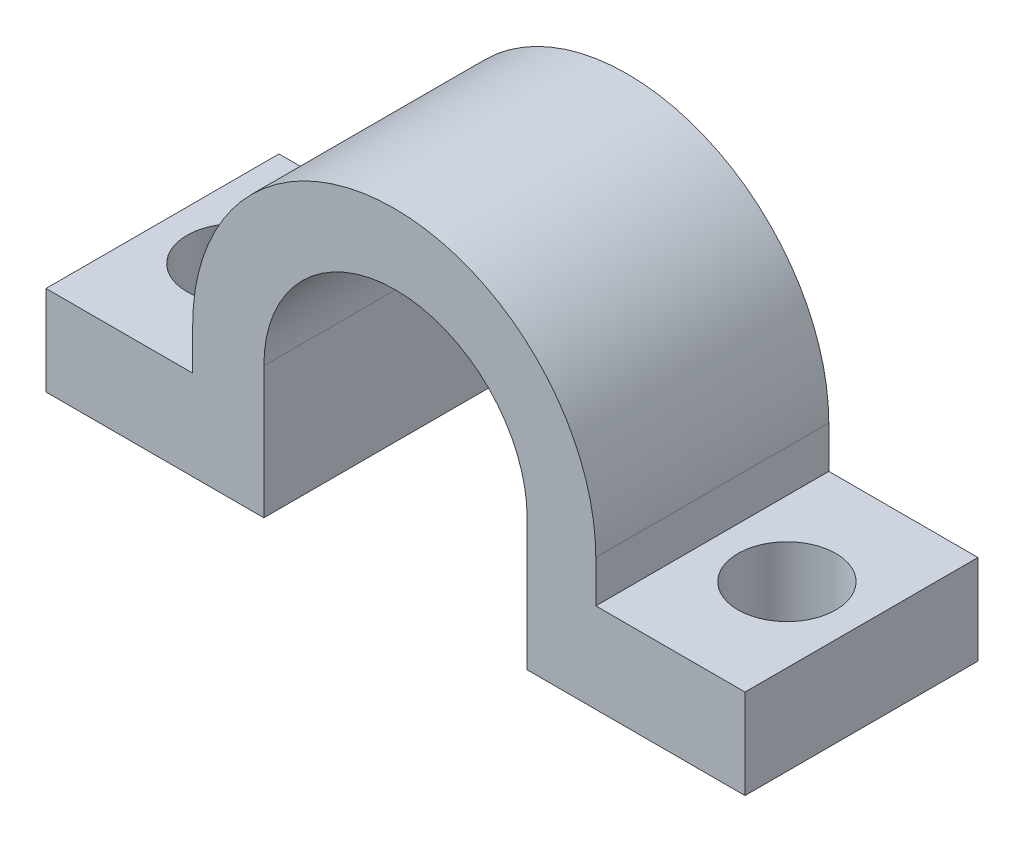
SolidWorks part; units mm, degrees
ref_plane "前视基准面" through (0, 0, 0) normal (0, 0, 1) x (1, 0, 0)
ref_plane "上视基准面" through (0, 0, 0) normal (0, 1, 0) x (1, 0, 0)
ref_plane "右视基准面" through (0, 0, 0) normal (1, 0, 0) x (0, 0, -1)
sketch "草图1" plane through (0, 0, 0) normal (0, 0, 1) x (1, 0, 0)
  line L0 (-5.5967, 5.1851) -> (-5.5967, 6.9851)
  line L13 (-14.9467, 5.1851) -> (-8.65, 5.1851)
  line L14 (-14.9467, 5.1851) -> (-14.9467, 1.3351)
  line L15 (-14.9467, 1.3351) -> (-5.5967, 1.3351)
  line L16 (-5.5967, 5.1851) -> (-5.5967, 1.3351)
  line L17 (8.65, 5.1851) -> (15.0533, 5.1851)
  line L18 (5.7033, 5.1851) -> (5.7033, 1.3351)
  line L19 (5.7033, 1.3351) -> (15.0533, 1.3351)
  line L20 (15.0533, 5.1851) -> (15.0533, 1.3351)
  line L22 (5.7033, 6.9851) -> (5.7033, 5.1851)
  line L23 (-8.65, 6.9851) -> (-8.65, 5.1851)
  line L24 (8.65, 6.9851) -> (8.65, 5.1851)
  arc A3 (8.65, 6.9851) -> (-8.65, 6.9851) centre (0, 6.9851) ccw
  arc A4 (5.7033, 6.9851) -> (-5.5967, 6.9851) centre (0.0533, 6.9851) ccw
  dimension "D1" = 3.85
  dimension "D8" = 11.3
  dimension "D2" = 3.85
  dimension "D3" = 0
  dimension "D4" = 11.3
  dimension "D6" = 9.35
  dimension "D7" = 30
extrude "凸台-拉伸1" add sketch "草图1" along normal blind 10
extrude "切除-拉伸1" cut sketch "草图2" against normal up to surface (17.7 mm away)
sketch "草图2" plane through (-970.0906, 5.1851, 1019.2503) normal (0, 1, 0) x (0, 0, 1)
  line L0 (-1055.2503, 985.1439) -> (-1055.2503, 955.1439) construction
  line L3 (-1014.2503, 985.1439) -> (-1014.2503, 955.1439) construction
  line L6 (-1060.2503, 981.9423) -> (-1009.2503, 981.9423) construction
  line L9 (-1060.2503, 958.2923) -> (-1009.2503, 958.2923) construction
  circle A0 centre (-1055.2503, 981.9423) radius 2.1
  circle A1 centre (-1055.2503, 958.2923) radius 2.1
  circle A2 centre (-1014.2503, 958.2923) radius 2.1
  circle A3 centre (-1014.2503, 981.9423) radius 2.1
sketch "草图7" plane through (0, 5.1851, 0) normal (0, 1, 0) x (1, 0, 0)
  circle A0 centre (-11.7983, -5) radius 2.1
  circle A1 centre (11.8517, -5) radius 2.1
